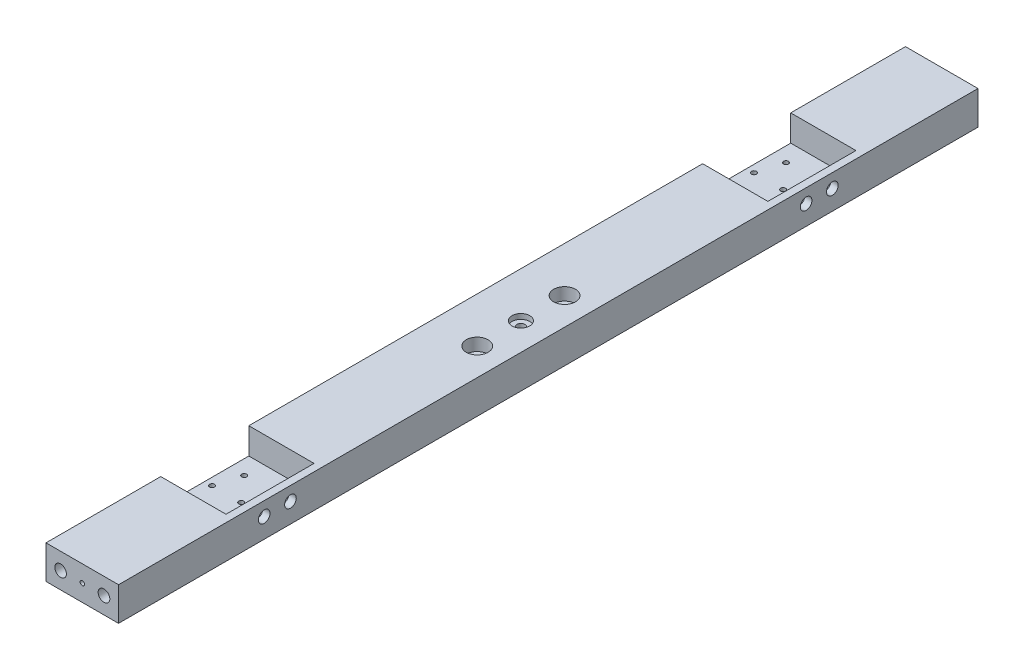
from build123d import *

# Parameters (mm, degrees)
SKETCH1_W                                           = 40
SKETCH1_H                                           = 590
BOSS_EXTRUDE1_DEPTH                                 = 23
CBORE_FOR_M8_HEX_SOCKET_HEAD_CAP_SCREW0_D           = 9
CBORE_FOR_M8_HEX_SOCKET_HEAD_CAP_SCREW0_DEPTH       = 41.94
CBORE_FOR_M8_HEX_SOCKET_HEAD_CAP_SCREW0_CBORE_D     = 15
CBORE_FOR_M8_HEX_SOCKET_HEAD_CAP_SCREW0_CBORE_DEPTH = 8.6
CBORE_FOR_M8_HEX_SOCKET_HEAD_CAP_SCREW0_TIP         = 2.703872786
SKETCH9_W                                           = 125.292505666
SKETCH9_H                                           = 60.455114524
CUT_EXTRUDE1_DEPTH                                  = 18
SKETCH11_W                                          = 4.8
SKETCH11_H                                          = 78.772442738
SKETCH11_H_2                                        = 311.544885476
BOSS_EXTRUDE2_DEPTH                                 = 23
SKETCH12_W                                          = 60.455114524
SKETCH12_H                                          = 5
BOSS_EXTRUDE3_DEPTH                                 = 4.8
SKETCH13_W                                          = 5
SKETCH13_H                                          = 590
BOSS_EXTRUDE4_DEPTH                                 = 23
SKETCH14_R                                          = 4
CUT_EXTRUDE2_DEPTH                                  = 15
SKETCH15_R                                          = 1.7
CUT_EXTRUDE3_DEPTH                                  = 15
CBORE_FOR_M5_HEX_HEAD_BOLT1_D                       = 5.5
CBORE_FOR_M5_HEX_HEAD_BOLT1_DEPTH                   = 41.94
CBORE_FOR_M5_HEX_HEAD_BOLT1_CBORE_D                 = 12.238
CBORE_FOR_M5_HEX_HEAD_BOLT1_CBORE_DEPTH             = 3.5
CBORE_FOR_M5_HEX_HEAD_BOLT1_TIP                     = 1.652366702
F_8_0MM_DOWEL_HOLE1_D                               = 8
F_8_0MM_DOWEL_HOLE1_DEPTH                           = 41.94
F_8_0MM_DOWEL_HOLE1_TIP                             = 2.403442476
F_3_0MM_DOWEL_HOLE1_D                               = 3
F_3_0MM_DOWEL_HOLE1_DEPTH                           = 41.94
F_3_0MM_DOWEL_HOLE1_TIP                             = 0.901290929


with BuildPart() as part:
    # Sketch1 → Boss-Extrude1 (new body)
    with BuildSketch(Plane(origin=(0, 0, 0), x_dir=(1, 0, 0), z_dir=(0, 1, 0))):
        with Locations((-11, 0)):
            Rectangle(SKETCH1_W, SKETCH1_H)
    extrude(amount=BOSS_EXTRUDE1_DEPTH)

    # CBORE for M8 Hex Socket Head Cap Screw0
    with Locations(Plane(origin=(0, 23, 30), x_dir=(0, 0, 1), z_dir=(0, 1, 0))):
        with Locations((0, 0), (-60, 0)):
            CounterBoreHole(CBORE_FOR_M8_HEX_SOCKET_HEAD_CAP_SCREW0_D / 2, CBORE_FOR_M8_HEX_SOCKET_HEAD_CAP_SCREW0_CBORE_D / 2, CBORE_FOR_M8_HEX_SOCKET_HEAD_CAP_SCREW0_CBORE_DEPTH, depth=CBORE_FOR_M8_HEX_SOCKET_HEAD_CAP_SCREW0_DEPTH)
            with Locations((0, 0, -(CBORE_FOR_M8_HEX_SOCKET_HEAD_CAP_SCREW0_DEPTH + CBORE_FOR_M8_HEX_SOCKET_HEAD_CAP_SCREW0_TIP / 2))):  # 118° drill point
                Cone(0, CBORE_FOR_M8_HEX_SOCKET_HEAD_CAP_SCREW0_D / 2, CBORE_FOR_M8_HEX_SOCKET_HEAD_CAP_SCREW0_TIP, mode=Mode.SUBTRACT)

    # Sketch9 → Cut-Extrude1 (cut)
    with BuildSketch(Plane(origin=(0, 23, 0), x_dir=(1, 0, 0), z_dir=(0, 1, 0))):
        with Locations((-26, -186)):
            Rectangle(SKETCH9_W, SKETCH9_H)
    cut_extrude1 = extrude(amount=-CUT_EXTRUDE1_DEPTH, mode=Mode.SUBTRACT)

    # Mirror1: Cut-Extrude1 across plane
    add(cut_extrude1.mirror(Plane.XY), mode=Mode.SUBTRACT)

    # Sketch11 → Boss-Extrude2 (add)
    with BuildSketch(Plane(origin=(0, 23, 0), x_dir=(1, 0, 0), z_dir=(0, 1, 0))):
        with Locations((11.4, -255.613778631)):
            Rectangle(SKETCH11_W, SKETCH11_H)
        with Locations((11.4, 255.613778631)):
            Rectangle(SKETCH11_W, SKETCH11_H)
        with Locations((11.4, 0)):
            Rectangle(SKETCH11_W, SKETCH11_H_2)
    extrude(amount=-BOSS_EXTRUDE2_DEPTH)

    # Sketch12 → Boss-Extrude3 (add)
    with BuildSketch(Plane(origin=(9, 0, 0), x_dir=(0, 0, -1), z_dir=(1, 0, 0))):
        with Locations((-186, 2.5)):
            Rectangle(SKETCH12_W, SKETCH12_H)
    boss_extrude3 = extrude(amount=BOSS_EXTRUDE3_DEPTH)

    # Mirror2: Boss-Extrude3 across plane
    add(boss_extrude3.mirror(Plane.XY))

    # Sketch13 → Boss-Extrude4 (add)
    with BuildSketch(Plane(origin=(0, 23, 0), x_dir=(1, 0, 0), z_dir=(0, 1, 0))):
        with Locations((16.3, 0)):
            Rectangle(SKETCH13_W, SKETCH13_H)
    extrude(amount=-BOSS_EXTRUDE4_DEPTH)

    # Sketch14 → Cut-Extrude2 (cut)
    with BuildSketch(Plane(origin=(18.8, 0, 0), x_dir=(0, 0, -1), z_dir=(1, 0, 0))):
        with Locations((-195, 13.5)):
            Circle(SKETCH14_R)
        with Locations((-177, 13.5)):
            Circle(SKETCH14_R)
    cut_extrude2 = extrude(amount=-CUT_EXTRUDE2_DEPTH, mode=Mode.SUBTRACT)

    # Mirror3: Cut-Extrude2 across plane
    add(cut_extrude2.mirror(Plane.XY), mode=Mode.SUBTRACT)

    # Sketch15 → Cut-Extrude3 (cut)
    with BuildSketch(Plane(origin=(0, 5, 0), x_dir=(1, 0, 0), z_dir=(0, 1, 0))):
        with Locations(Location((-21, -169, 0), (0, 0, 270))):
            Circle(SKETCH15_R)
        with Locations(Location((-6, -186, 0), (0, 0, 270))):
            Circle(SKETCH15_R)
        with Locations(Location((-26, -186, 0), (0, 0, 270))):
            Circle(SKETCH15_R)
        with Locations(Location((-21, -203, 0), (0, 0, 270))):
            Circle(SKETCH15_R)
    cut_extrude3 = extrude(amount=-CUT_EXTRUDE3_DEPTH, mode=Mode.SUBTRACT)

    # Mirror4: Cut-Extrude3 across plane
    add(cut_extrude3.mirror(Plane.XY), mode=Mode.SUBTRACT)

    # CBORE for M5 Hex Head Bolt1
    with Locations(Plane.ZX.offset(23)):
        with Locations((0, 0)):
            CounterBoreHole(CBORE_FOR_M5_HEX_HEAD_BOLT1_D / 2, CBORE_FOR_M5_HEX_HEAD_BOLT1_CBORE_D / 2, CBORE_FOR_M5_HEX_HEAD_BOLT1_CBORE_DEPTH, depth=CBORE_FOR_M5_HEX_HEAD_BOLT1_DEPTH)
            with Locations((0, 0, -(CBORE_FOR_M5_HEX_HEAD_BOLT1_DEPTH + CBORE_FOR_M5_HEX_HEAD_BOLT1_TIP / 2))):  # 118° drill point
                Cone(0, CBORE_FOR_M5_HEX_HEAD_BOLT1_D / 2, CBORE_FOR_M5_HEX_HEAD_BOLT1_TIP, mode=Mode.SUBTRACT)

    # Ø8.0mm Dowel Hole1
    with Locations(Plane(origin=(-21, 11.5, 295), x_dir=(1, 0, 0), z_dir=(0, 0, 1))):
        with Locations((0, 0), (29.8, 0)):
            Hole(F_8_0MM_DOWEL_HOLE1_D / 2, depth=F_8_0MM_DOWEL_HOLE1_DEPTH)
            with Locations((0, 0, -(F_8_0MM_DOWEL_HOLE1_DEPTH + F_8_0MM_DOWEL_HOLE1_TIP / 2))):  # 118° drill point
                Cone(0, F_8_0MM_DOWEL_HOLE1_D / 2, F_8_0MM_DOWEL_HOLE1_TIP, mode=Mode.SUBTRACT)

    # Ø3.0mm Dowel Hole1
    with Locations(Plane(origin=(-6.1, 11.5, 295), x_dir=(1, 0, 0), z_dir=(0, 0, 1))):
        with Locations((0, 0)):
            Hole(F_3_0MM_DOWEL_HOLE1_D / 2, depth=F_3_0MM_DOWEL_HOLE1_DEPTH)
            with Locations((0, 0, -(F_3_0MM_DOWEL_HOLE1_DEPTH + F_3_0MM_DOWEL_HOLE1_TIP / 2))):  # 118° drill point
                Cone(0, F_3_0MM_DOWEL_HOLE1_D / 2, F_3_0MM_DOWEL_HOLE1_TIP, mode=Mode.SUBTRACT)


solid = part.part
